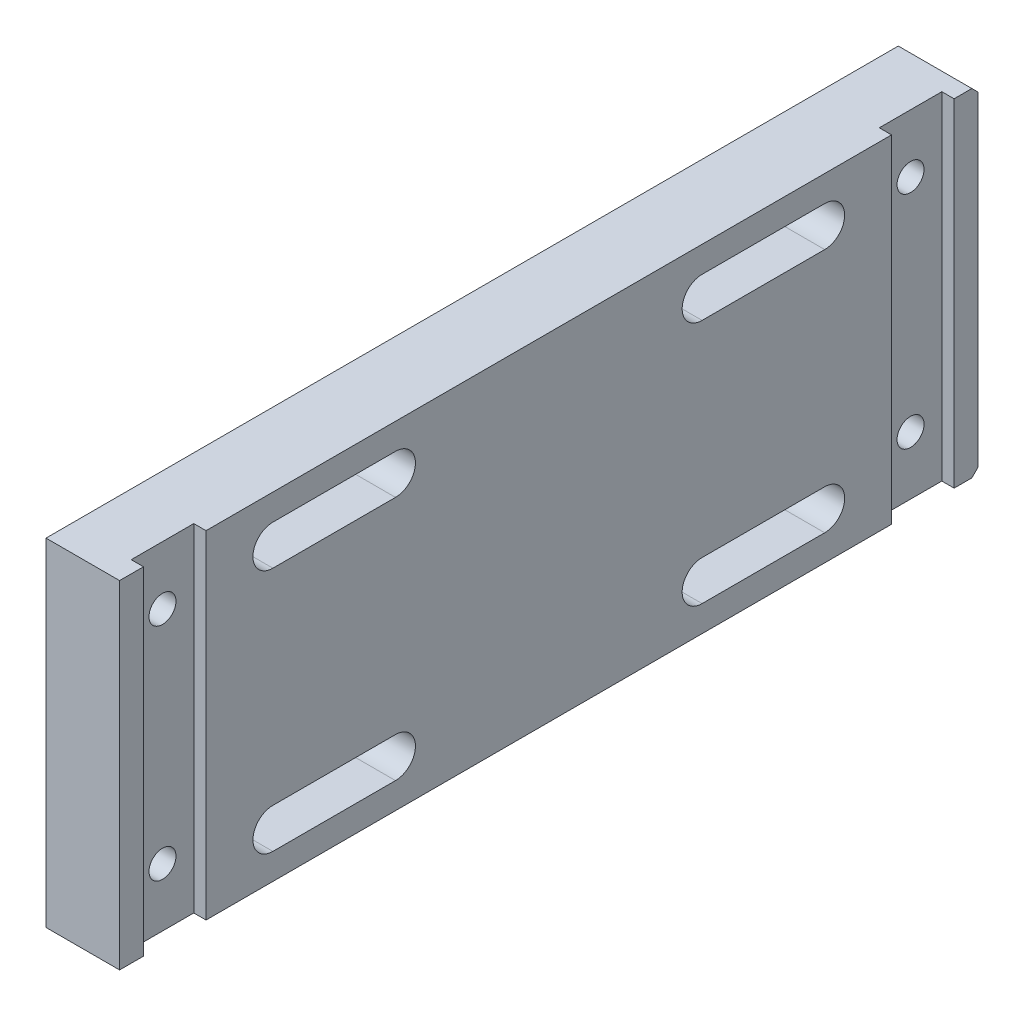
from build123d import *

# Parameters (mm, degrees)
SKETCH_1_W                = 140
SKETCH_1_H                = 55
EXTRUDE_1_DEPTH           = 12
SKETCH_2_W                = 10.2
SKETCH_2_H                = 67.741828953
CUT_EXTRUDE_1_DEPTH       = 2
CHAMFER_1_SIZE            = 1
CUT_EXTRUDE_2_DEPTH       = 36
HOLE_WIZARD_0_D           = 4.4
HOLE_WIZARD_0_CBORE_D     = 8
HOLE_WIZARD_0_CBORE_DEPTH = 5


with BuildPart() as part:
    # 草图1 → 凸台-拉伸1 (new body)
    with BuildSketch(Plane(origin=(0, 0, 0), x_dir=(0, 0, -1), z_dir=(1, 0, 0))):
        Rectangle(SKETCH_1_W, SKETCH_1_H)
    extrude(amount=EXTRUDE_1_DEPTH)

    # 草图2 → 切除-拉伸1 (cut)
    with BuildSketch(Plane(origin=(12, 0, 0), x_dir=(0, 0, -1), z_dir=(1, 0, 0))):
        with Locations((-61, -0.529795054)):
            Rectangle(SKETCH_2_W, SKETCH_2_H)
    cut_extrude_1 = extrude(amount=-CUT_EXTRUDE_1_DEPTH, mode=Mode.SUBTRACT)

    # 倒角1
    chamfer_1_edges = [part.edges().sort_by_distance(p)[0] for p in [
        (6, -27.5, -70),
        (6, 27.5, -70),
    ]]
    chamfer(chamfer_1_edges, length=CHAMFER_1_SIZE)

    # 镜向2: 切除-拉伸1 across plane
    add(cut_extrude_1.mirror(Plane.XY), mode=Mode.SUBTRACT)

    # 草图3 → 切除-拉伸2 (cut)
    with BuildSketch(Plane(origin=(12, 0, 0), x_dir=(0, 0, -1), z_dir=(1, 0, 0))):
        with BuildLine():
            Line((-45, 23.25), (-25, 23.25))
            ThreePointArc((-25, 23.25), (-21.75, 20), (-25, 16.75))
            Line((-25, 16.75), (-45, 16.75))
            ThreePointArc((-45, 16.75), (-48.25, 20), (-45, 23.25))
        make_face()
        with BuildLine():
            Line((-45, -23.25), (-25, -23.25))
            ThreePointArc((-25, -23.25), (-21.75, -20), (-25, -16.75))
            Line((-25, -16.75), (-45, -16.75))
            ThreePointArc((-45, -16.75), (-48.25, -20), (-45, -23.25))
        make_face()
        with BuildLine():
            Line((45, 23.25), (25, 23.25))
            ThreePointArc((25, 23.25), (21.75, 20), (25, 16.75))
            Line((25, 16.75), (45, 16.75))
            ThreePointArc((45, 16.75), (48.25, 20), (45, 23.25))
        make_face()
        with BuildLine():
            Line((45, -23.25), (25, -23.25))
            ThreePointArc((25, -23.25), (21.75, -20), (25, -16.75))
            Line((25, -16.75), (45, -16.75))
            ThreePointArc((45, -16.75), (48.25, -20), (45, -23.25))
        make_face()
    extrude(amount=-CUT_EXTRUDE_2_DEPTH, mode=Mode.SUBTRACT)

    # 打孔尺寸(%根据)内六角圆柱头螺钉的类型0 (through all)
    with Locations(Plane.ZY):
        with Locations((-61, 18), (-61, -18), (61, 18), (61, -18)):
            CounterBoreHole(HOLE_WIZARD_0_D / 2, HOLE_WIZARD_0_CBORE_D / 2, HOLE_WIZARD_0_CBORE_DEPTH)


solid = part.part
